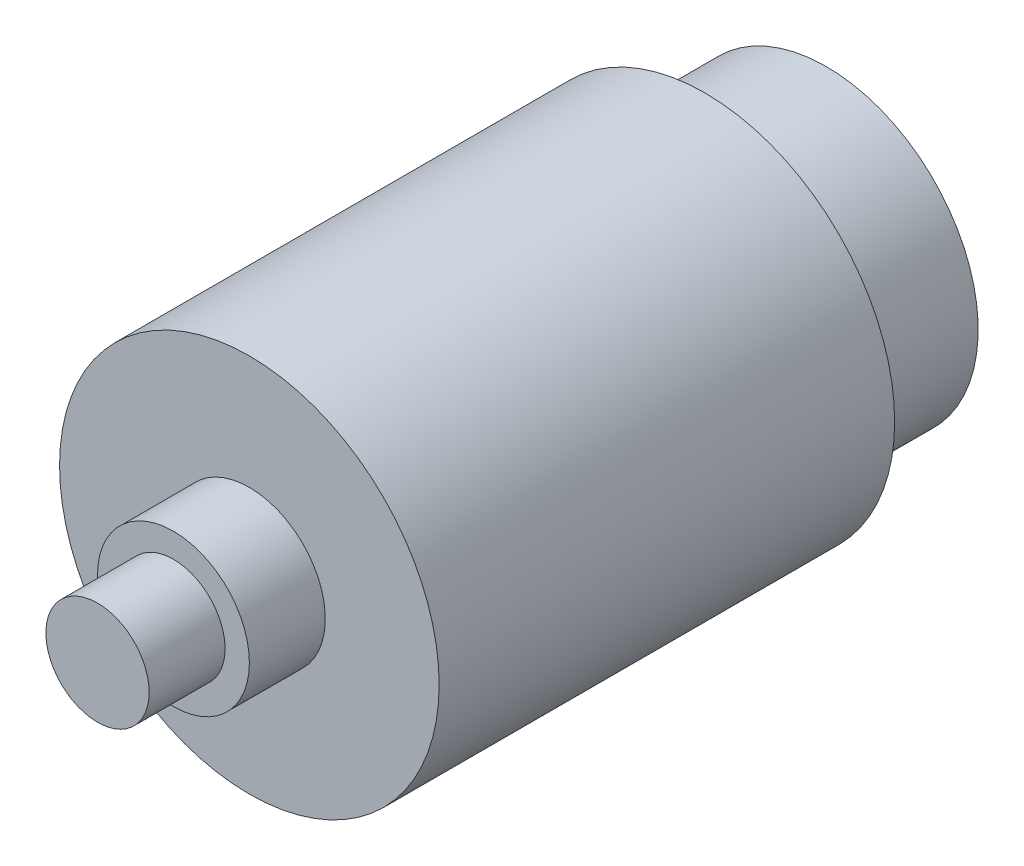
SolidWorks part; units mm, degrees
ref_plane "Front Plane" through (0, 0, 0) normal (0, 0, 1) x (1, 0, 0)
ref_plane "Top Plane" through (0, 0, 0) normal (0, 1, 0) x (1, 0, 0)
ref_plane "Right Plane" through (0, 0, 0) normal (1, 0, 0) x (0, 0, -1)
sketch "Sketch1" plane through (0, 0, 0) normal (0, 0, 1) x (1, 0, 0)
  circle A0 centre (0, 0) radius 5
  dimension "D1" = 10
extrude "Boss-Extrude1" add sketch "Sketch1" along normal blind 5
sketch "Sketch2" plane through (0, 0, 5) normal (0, 0, 1) x (1, 0, 0)
  circle A0 centre (0, 0) radius 3.4
  dimension "D1" = 6.8
extrude "Boss-Extrude2" add sketch "Sketch2" along normal blind 5
sketch "Sketch3" plane through (0, 0, 0) normal (0, 0, -1) x (-1, 0, 0)
  circle A0 centre (0, 0) radius 12.5
extrude "Boss-Extrude3" add sketch "Sketch3" along normal blind 30
sketch "Sketch4" plane through (0, 0, -30) normal (0, 0, -1) x (-1, 0, 0)
  circle A0 centre (0, 0) radius 10
extrude "Boss-Extrude4" add sketch "Sketch4" along normal blind 8
